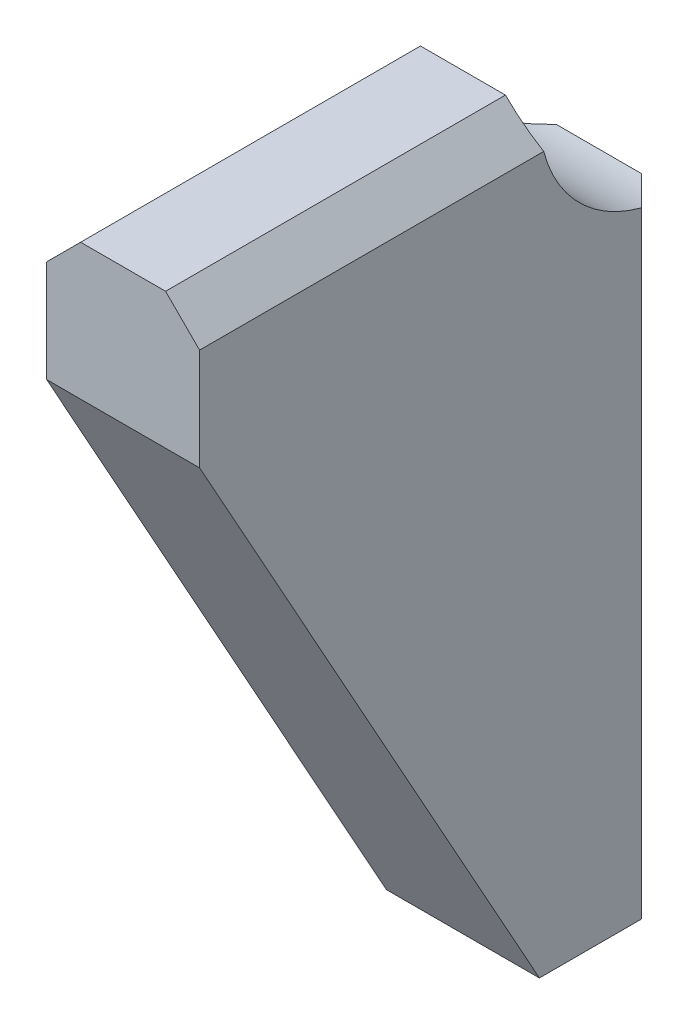
from build123d import *

# Parameters (mm, degrees)
BOSS_EXTRUDE1_DEPTH = 22.5
CHAMFER1_SIZE       = 10


with BuildPart() as part:
    # Sketch1 → Boss-Extrude1 (new, symmetric)
    with BuildSketch(Plane(origin=(0, 0, 0), x_dir=(0, 0, -1), z_dir=(1, 0, 0))):
        with BuildLine():
            Line((0, 0), (0, 180))
            ThreePointArc((0, 180), (-28.284271247, 191.715728753), (-40, 220))
            Line((-40, 220), (-140, 220))
            Line((-140, 220), (-140, 180))
            Line((-140, 180), (-40, 0))
            Line((-40, 0), (0, 0))
        make_face()
    extrude(amount=BOSS_EXTRUDE1_DEPTH, both=True)

    # Chamfer1
    chamfer1_edges = [part.edges().sort_by_distance(p)[0] for p in [
        (22.5, 220, 90),
        (-22.5, 220, 90),
        (22.5, 90, 0),
        (-22.5, 90, 0),
    ]]
    chamfer(chamfer1_edges, length=CHAMFER1_SIZE)


solid = part.part
